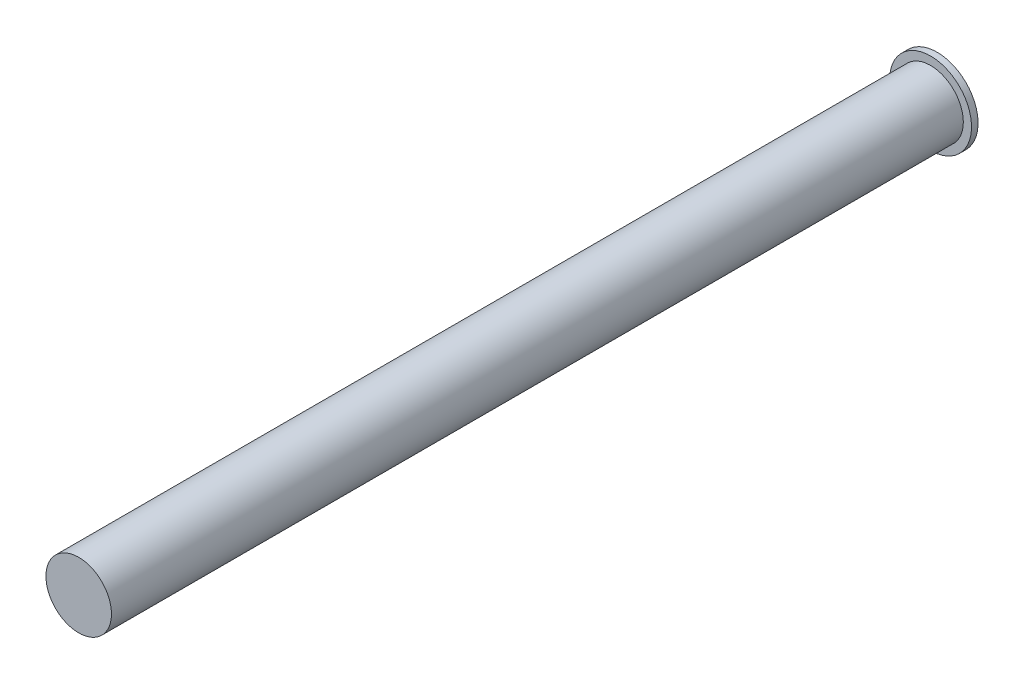
SolidWorks part; units mm, degrees
ref_plane "前视基准面" through (0, 0, 0) normal (0, 0, 1) x (1, 0, 0)
ref_plane "上视基准面" through (0, 0, 0) normal (0, 1, 0) x (1, 0, 0)
ref_plane "右视基准面" through (0, 0, 0) normal (1, 0, 0) x (0, 0, -1)
sketch "草图1" plane through (0, 0, 0) normal (0, 0, 1) x (1, 0, 0)
  circle A0 centre (0, 0) radius 5
  dimension "D1" = 10
extrude "凸台-拉伸1" add sketch "草图1" along normal blind 130
sketch "草图2" plane through (0, 0, 0) normal (0, 0, -1) x (-1, 0, 0)
  circle A0 centre (0, 0) radius 6.25
  dimension "D1" = 12.5
extrude "凸台-拉伸2" add sketch "草图2" along normal blind 1
